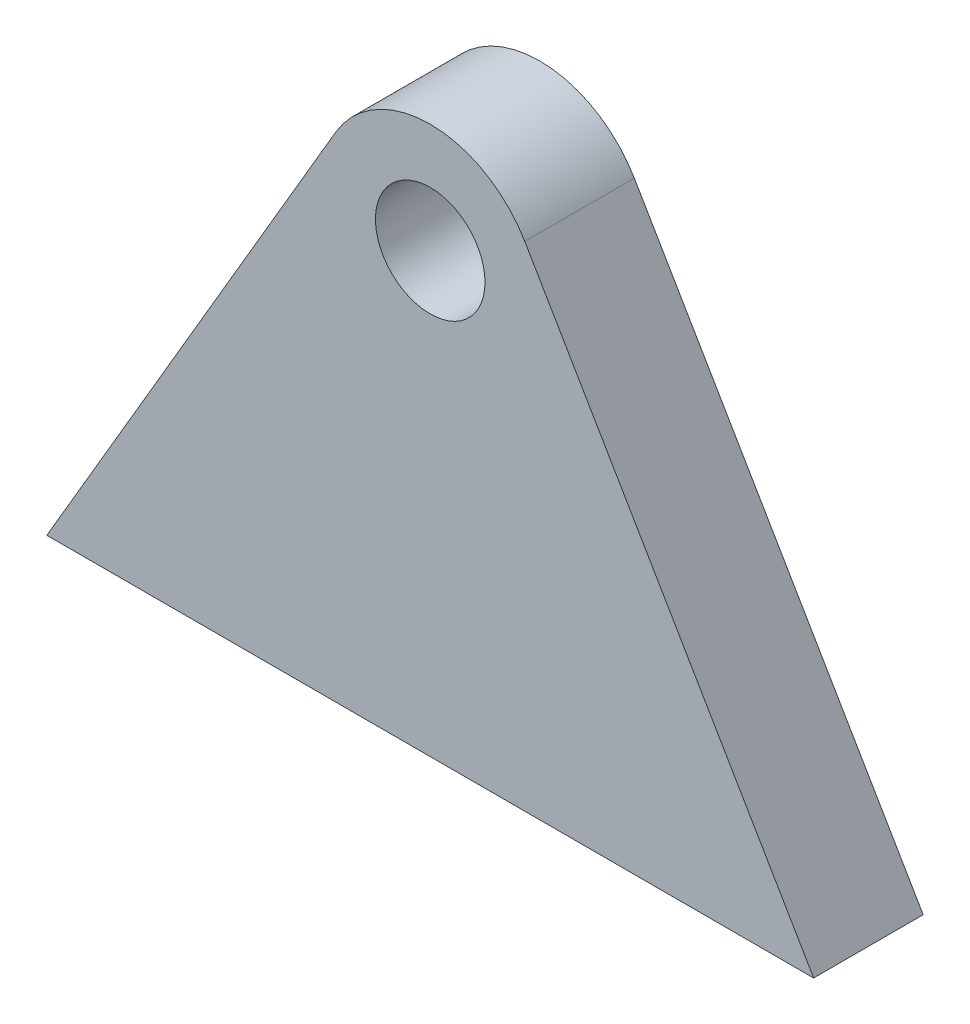
from build123d import *

# Parameters (mm, degrees)
SKETCH1_R           = 5
BOSS_EXTRUDE1_DEPTH = 10


with BuildPart() as part:
    # Sketch1 → Boss-Extrude1 (new body)
    with BuildSketch(Plane.XY):
        with BuildLine():
            Line((-35, -40), (35, -40))
            Line((35, -40), (8.630305493, 5.051517306))
            ThreePointArc((8.630305493, 5.051517306), (0, 10), (-8.630305493, 5.051517306))
            Line((-8.630305493, 5.051517306), (-35, -40))
        make_face()
        Circle(SKETCH1_R, mode=Mode.SUBTRACT)
    extrude(amount=BOSS_EXTRUDE1_DEPTH)


solid = part.part
